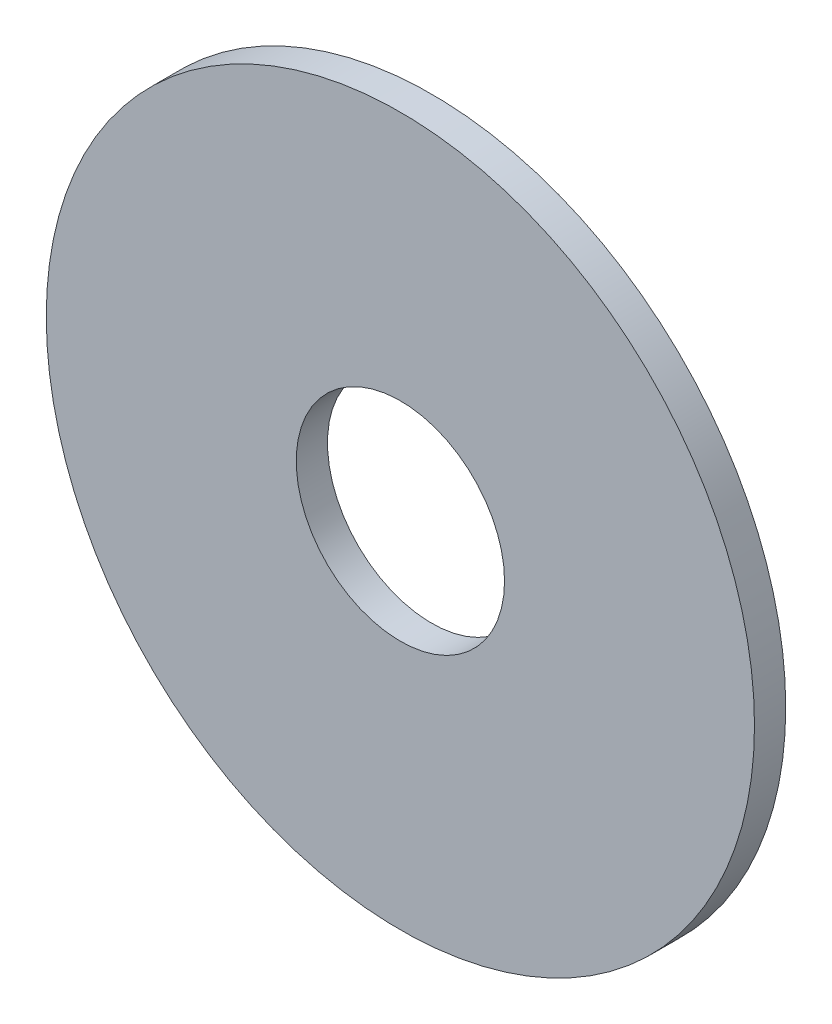
from build123d import *

# Parameters (mm, degrees)
SKETCH1_R               = 85
BOSS_EXTRUDE1_DEPTH     = 7.5
CUT_EXTRUDE1_DEPTH      = 121.441894704
CUT_EXTRUDE1_DEPTH_BACK = 121.441894704
SKETCH2_R               = 25


with BuildPart() as part:
    # Sketch1 → Boss-Extrude1 (new body)
    with BuildSketch(Plane.XY):
        Circle(SKETCH1_R)
    extrude(amount=BOSS_EXTRUDE1_DEPTH)

    # Sketch2 → Cut-Extrude1 (cut, two sides: drawn at the far end of the back side and taken through both)
    with BuildSketch(Plane.XY.offset(7.5).offset(-CUT_EXTRUDE1_DEPTH_BACK)):
        Circle(SKETCH2_R)
    extrude(amount=CUT_EXTRUDE1_DEPTH + CUT_EXTRUDE1_DEPTH_BACK, mode=Mode.SUBTRACT)


solid = part.part
